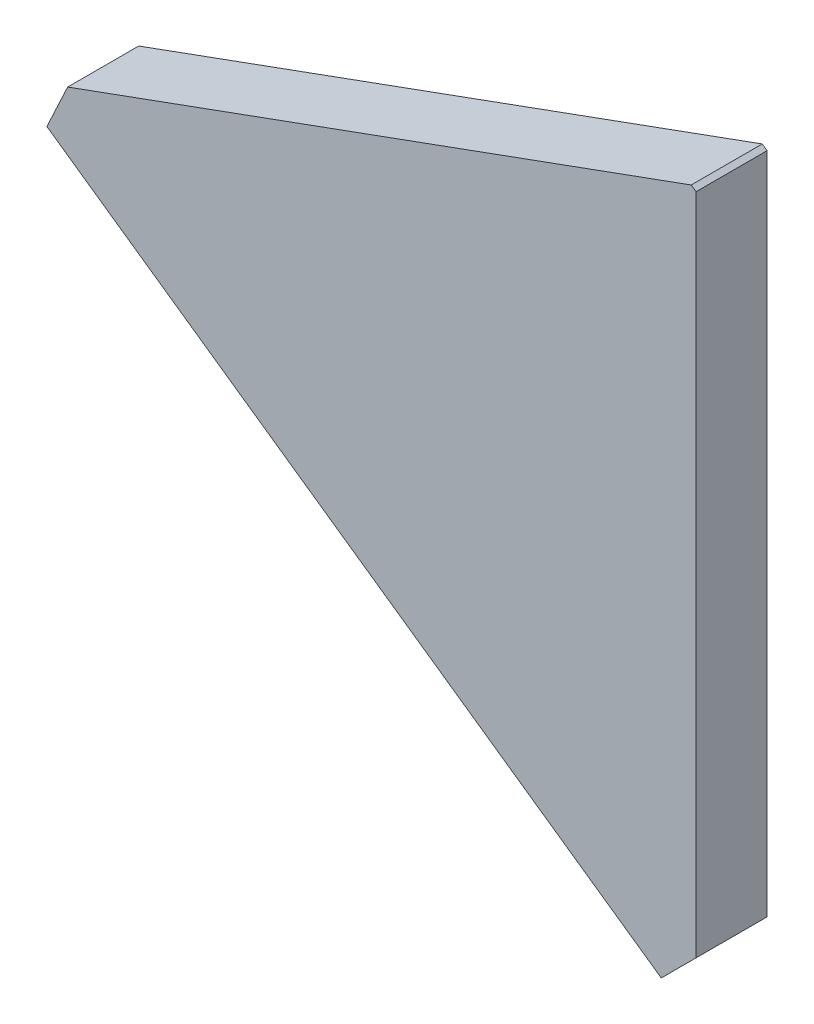
SolidWorks part; units mm, degrees
material "Q235-A "
ref_plane "前视基准面" through (0, 0, 0) normal (0, 0, 1) x (1, 0, 0)
ref_plane "上视基准面" through (0, 0, 0) normal (0, 1, 0) x (1, 0, 0)
ref_plane "右视基准面" through (0, 0, 0) normal (1, 0, 0) x (0, 0, -1)
sketch "草图1" plane through (0, 0, 0) normal (0, 0, 1) x (1, 0, 0)
  line L0 (-0.8192, 243.4328) -> (-115.5344, 201.6799)
  line L1 (-190.38, 174.4383) -> (-115.0144, 201.8692) construction
  line L2 (-115.5344, 201.6799) -> (0, 120.7818)
  line L3 (0, 41.1328) -> (0, 121.3353) construction
  line L4 (0, 120.7818) -> (0, 242.8593)
  line L7 (-0.8192, 243.4328) -> (0, 242.8593)
  dimension "D1" = 100
extrude "凸台-拉伸1" add sketch "草图1" along normal blind 12 from offset 260 offset against normal yes
chamfer "倒角1" distance 10 angle 45 2 edges at (0, 120.7818, -254) (-115.5344, 201.6799, -254)
